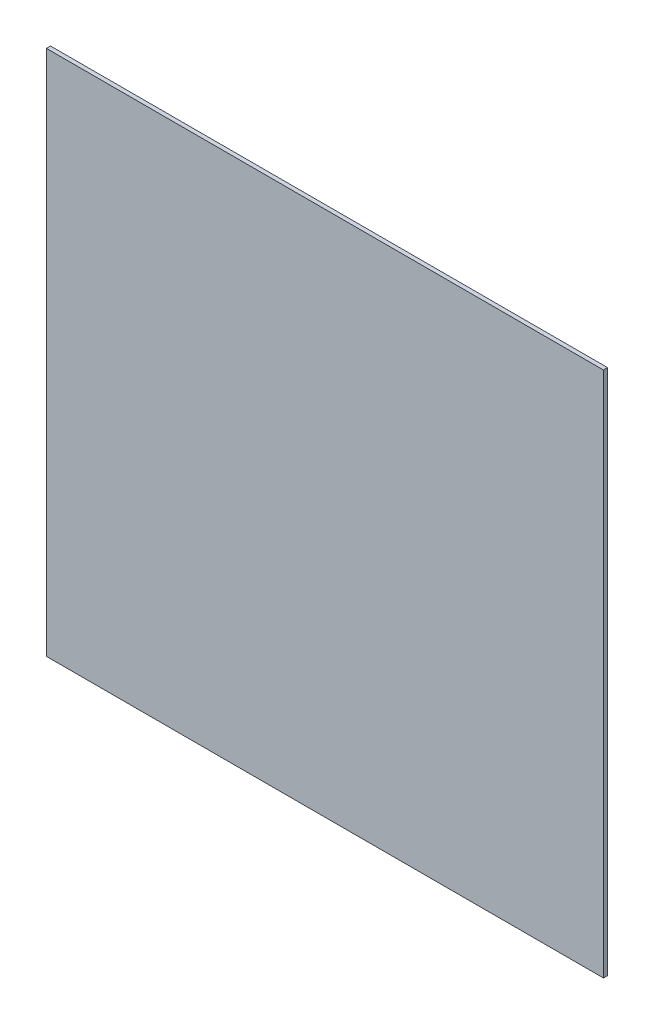
from build123d import *

# Parameters (mm, degrees)
SKETCH_1_W      = 676
SKETCH_1_H      = 639
EXTRUDE_1_DEPTH = 5


with BuildPart() as part:
    # 草图1 → 凸台-拉伸1 (new body)
    with BuildSketch(Plane.XY):
        Rectangle(SKETCH_1_W, SKETCH_1_H)
    extrude(amount=EXTRUDE_1_DEPTH)


solid = part.part
